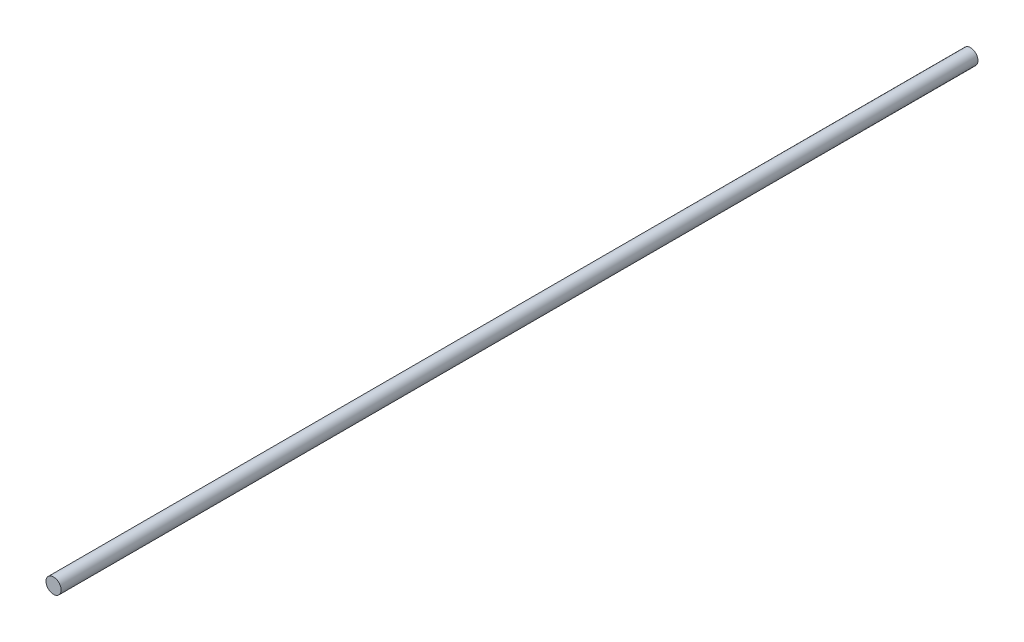
from build123d import *

# Parameters (mm, degrees)
SKETCH1_R           = 2
BOSS_EXTRUDE1_DEPTH = 242.5


with BuildPart() as part:
    # Sketch1 → Boss-Extrude1 (new body)
    with BuildSketch(Plane.XY):
        Circle(SKETCH1_R)
    extrude(amount=BOSS_EXTRUDE1_DEPTH)


solid = part.part
